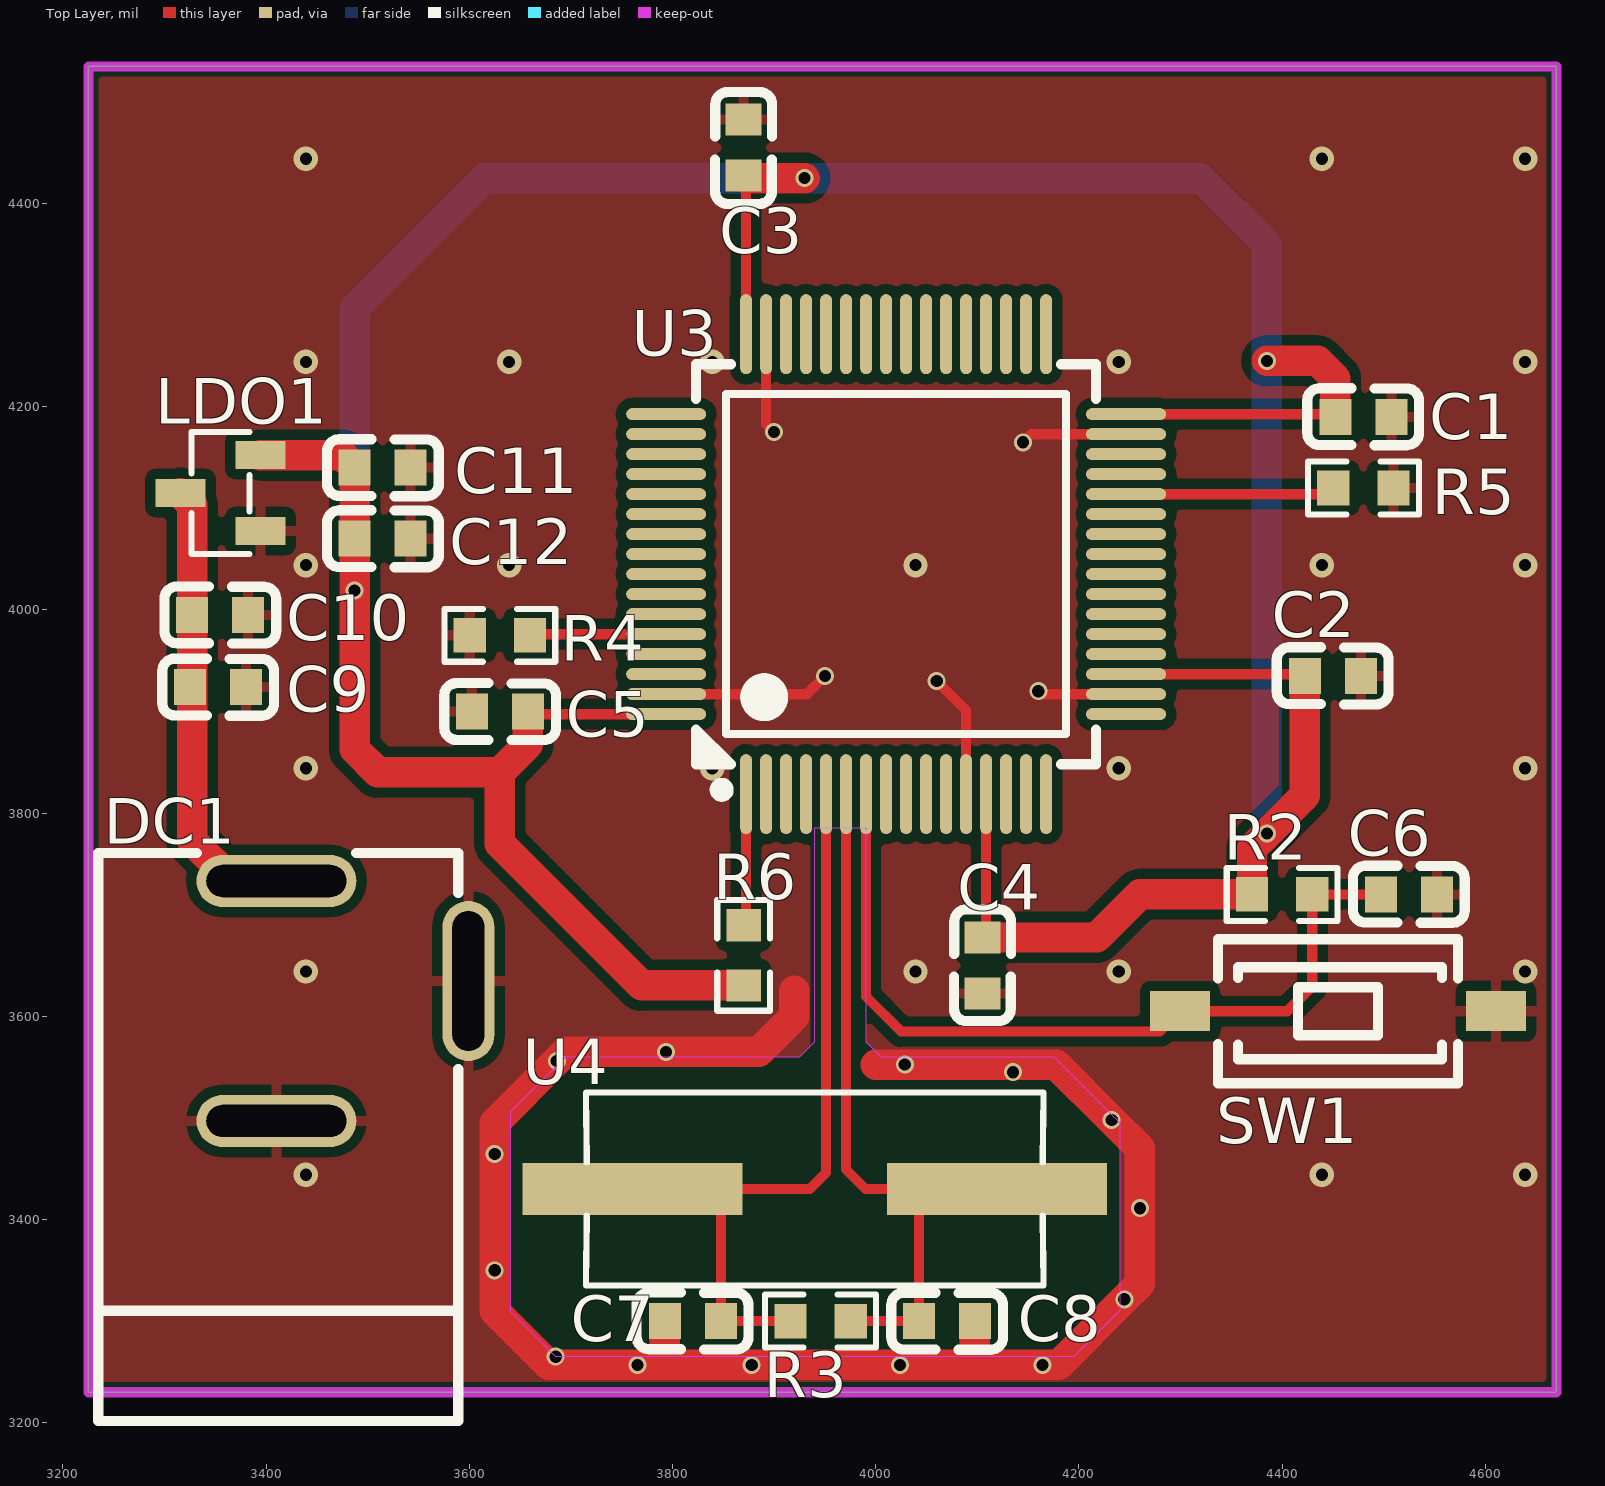
[diagram p0: Top Layer view]
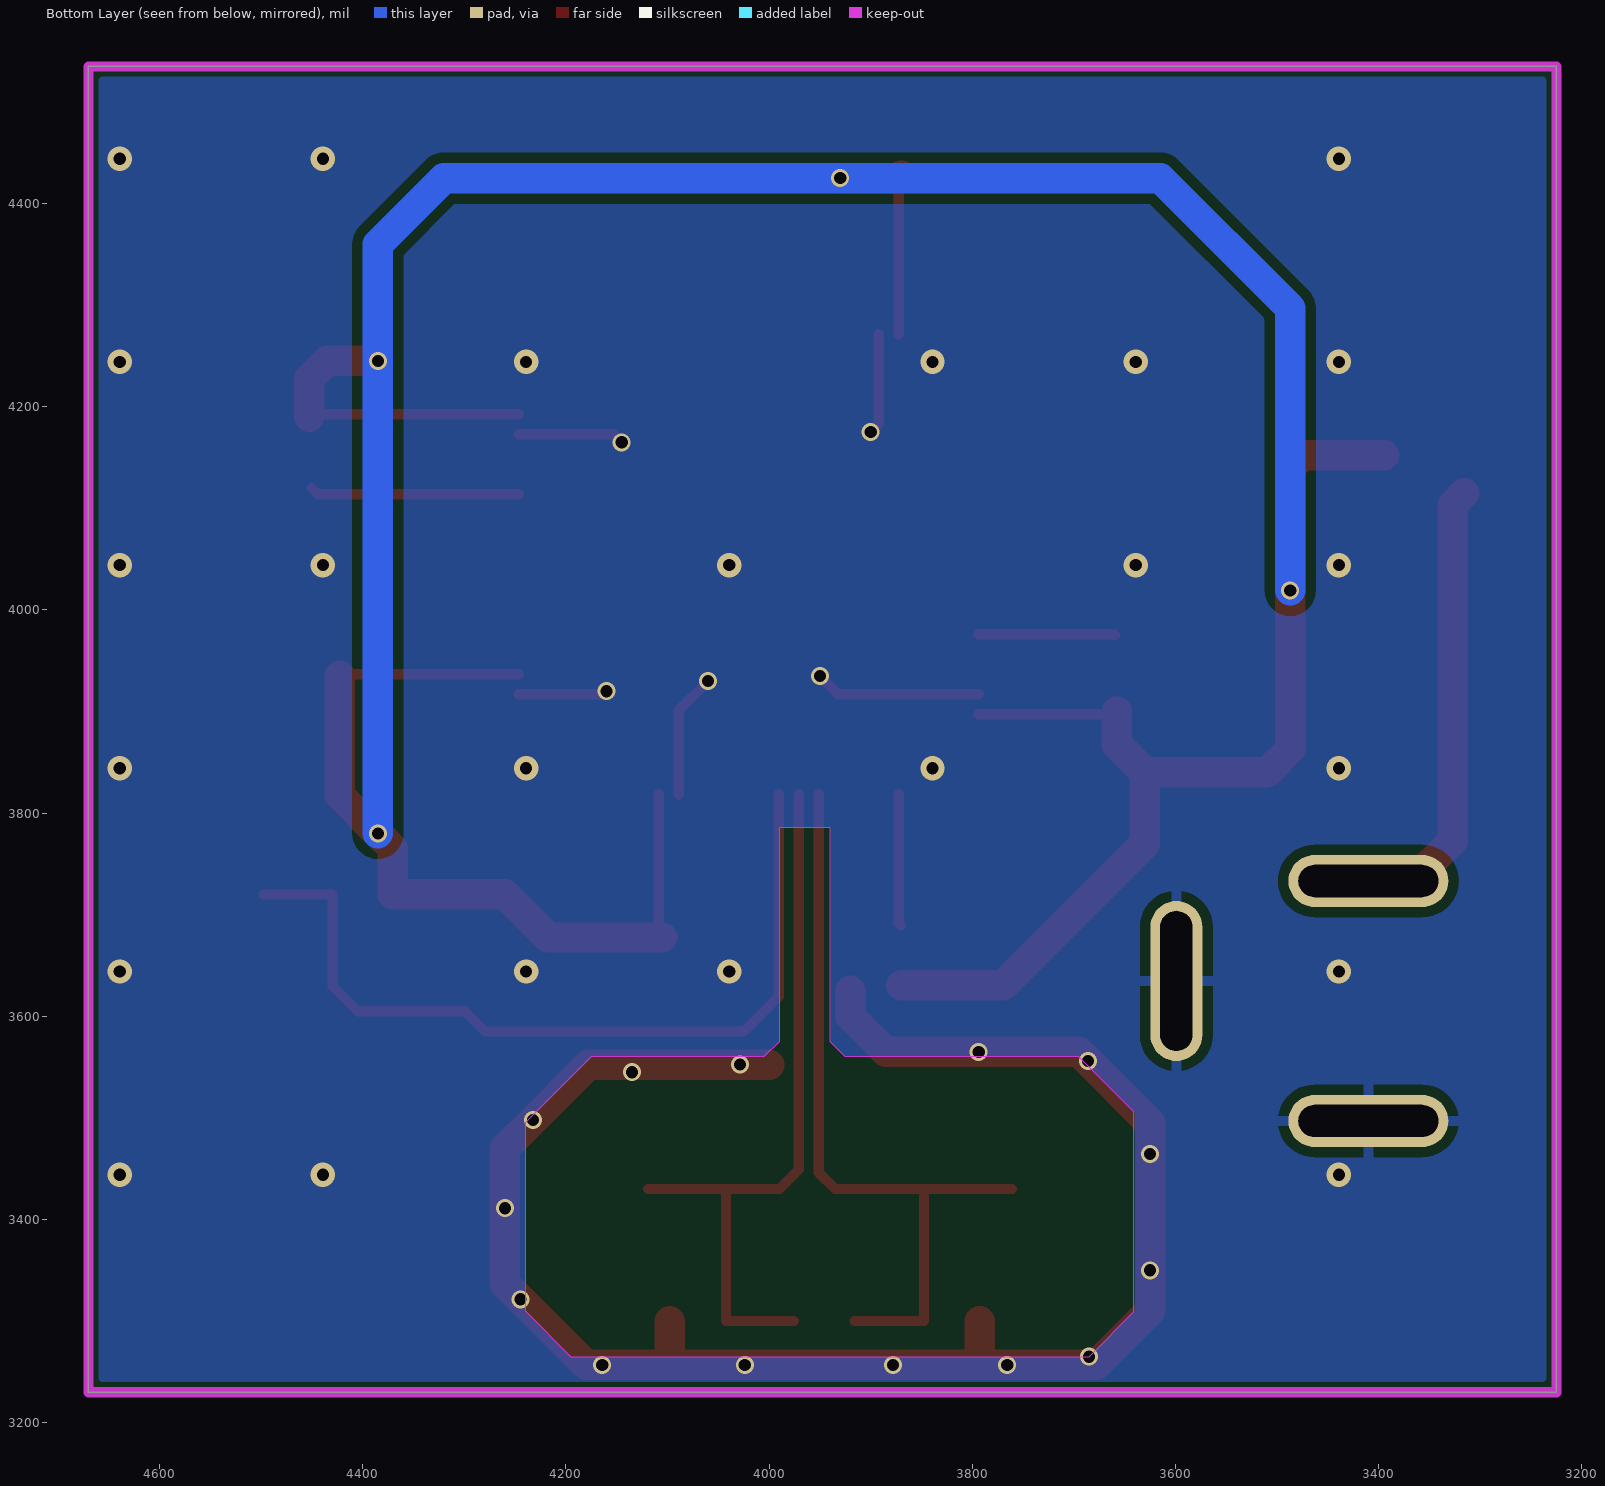
[diagram p1: Bottom Layer view, seen from below]
# Altium PCB MISC52126.pcbdoc
Units mil, origin at the board's own origin, x right, y up, seen from the top; angles counter-clockwise.
Board outline 1445 x 1305 mil, 2 copper layers (Top Layer, Bottom Layer), stack 62.206 mil thick; 22 components, 57 nets, 108 pads, 47 vias.

## Layer stack, top to bottom
Top Solder Mask Layer: solder mask 0.394, Dk 3.3
Top Layer: signal copper 1.379
Dielectric1: surface 59.449, FR4, Dk 4.5
Bottom Layer: signal copper 1.378
Bottom Solder Mask Layer: solder mask 0.394, Dk 3.3

## Board outline
3225,4535 3225,3230 4670,3230 4670,4535

## Design rules (kind name [scope] priority, off if disabled: settings)
BoardOutlineClearance copperThickness2oz_1 [All] p2 off: genericclearance=7.99 ignorepadtopadclearanceinfootprint=FALSE except(0: Arc-SplitContinuation Track-SplitContinuation SMDPad-SplitContinuation THPad-SplitContinuation Via-SplitContinuation Fill-SplitContinuation Region-SplitContinuation Poly-SplitContinuation Text-SplitContinuation Hole-SplitContinuation; 5.98: Arc-CutoutEdge Track-CutoutEdge SMDPad-CutoutEdge THPad-CutoutEdge Via-CutoutEdge Fill-CutoutEdge Region-CutoutEdge Text-CutoutEdge Hole-CutoutEdge; 10: Poly-OutlineEdge Poly-CutoutEdge; 11.81: Arc-OutlineEdge Track-OutlineEdge SMDPad-OutlineEdge THPad-OutlineEdge Via-OutlineEdge Fill-OutlineEdge Region-OutlineEdge Text-OutlineEdge Hole-OutlineEdge)
BoardOutlineClearance Plane_innerPlane_1 [All] p4 off: genericclearance=4.02 ignorepadtopadclearanceinfootprint=FALSE except(0: Arc-SplitContinuation Track-SplitContinuation SMDPad-SplitContinuation THPad-SplitContinuation Via-SplitContinuation Fill-SplitContinuation Region-SplitContinuation Poly-SplitContinuation Text-SplitContinuation Hole-SplitContinuation; 5.98: Arc-CutoutEdge Track-CutoutEdge SMDPad-CutoutEdge THPad-CutoutEdge Via-CutoutEdge Fill-CutoutEdge Region-CutoutEdge Text-CutoutEdge Hole-CutoutEdge; 10: Poly-OutlineEdge Poly-CutoutEdge; 11.81: Arc-OutlineEdge Track-OutlineEdge SMDPad-OutlineEdge THPad-OutlineEdge Via-OutlineEdge Fill-OutlineEdge Region-OutlineEdge Text-OutlineEdge Hole-OutlineEdge)
BoardOutlineClearance Copper_copperRegion_1 [All] p6 off: genericclearance=4.02 ignorepadtopadclearanceinfootprint=FALSE except(0: Arc-SplitContinuation Track-SplitContinuation SMDPad-SplitContinuation THPad-SplitContinuation Via-SplitContinuation Fill-SplitContinuation Region-SplitContinuation Poly-SplitContinuation Text-SplitContinuation Hole-SplitContinuation; 5.98: Arc-CutoutEdge Track-CutoutEdge SMDPad-CutoutEdge THPad-CutoutEdge Via-CutoutEdge Fill-CutoutEdge Region-CutoutEdge Text-CutoutEdge Hole-CutoutEdge; 10: Poly-OutlineEdge Poly-CutoutEdge; 11.81: Arc-OutlineEdge Track-OutlineEdge SMDPad-OutlineEdge THPad-OutlineEdge Via-OutlineEdge Fill-OutlineEdge Region-OutlineEdge Text-OutlineEdge Hole-OutlineEdge)
BoardOutlineClearance copperThickness1oz_1 [All] p8: genericclearance=4.02 ignorepadtopadclearanceinfootprint=FALSE except(0: Arc-SplitContinuation Track-SplitContinuation SMDPad-SplitContinuation THPad-SplitContinuation Via-SplitContinuation Fill-SplitContinuation Region-SplitContinuation Poly-SplitContinuation Text-SplitContinuation Hole-SplitContinuation; 5.98: Arc-CutoutEdge Track-CutoutEdge SMDPad-CutoutEdge THPad-CutoutEdge Via-CutoutEdge Fill-CutoutEdge Region-CutoutEdge Text-CutoutEdge Hole-CutoutEdge; 10: Poly-OutlineEdge Poly-CutoutEdge; 11.81: Arc-OutlineEdge Track-OutlineEdge SMDPad-OutlineEdge THPad-OutlineEdge Via-OutlineEdge Fill-OutlineEdge Region-OutlineEdge Text-OutlineEdge Hole-OutlineEdge)
Clearance copperThickness2oz [All] p1 off: gap=7.99 ignorepadtopadclearanceinfootprint=FALSE except(5.98: SMDPad-Track SMDPad-SMDPad THPad-Track SMDPad-THPad THPad-THPad Track-Via SMDPad-Via THPad-Via Via-Via Fill-Track Region-Track Fill-SMDPad Region-SMDPad Fill-THPad Region-THPad Fill-Via Region-Via Fill-Fill Fill-Region Region-Region Arc-Track Arc-SMDPad Arc-THPad Arc-Via Fill-Arc Region-Arc Arc-Arc Text-Track SMDPad-Text Text-THPad Text-Via Fill-Text Region-Text Arc-Text Text-Text Hole-Track Hole-SMDPad Hole-THPad Hole-Via Fill-Hole Region-Hole Hole-Arc Hole-Text; 10: Poly-Track Poly-SMDPad Poly-THPad Poly-Via Poly-Fill Poly-Region Poly-Poly Poly-Arc Poly-Text Poly-Hole)
Clearance Plane_innerPlane [All] p3 off: gap=4.02 ignorepadtopadclearanceinfootprint=FALSE except(5.98: SMDPad-Track SMDPad-SMDPad THPad-Track SMDPad-THPad THPad-THPad Track-Via SMDPad-Via THPad-Via Via-Via Fill-Track Region-Track Fill-SMDPad Region-SMDPad Fill-THPad Region-THPad Fill-Via Region-Via Fill-Fill Fill-Region Region-Region Arc-Track Arc-SMDPad Arc-THPad Arc-Via Fill-Arc Region-Arc Arc-Arc Text-Track SMDPad-Text Text-THPad Text-Via Fill-Text Region-Text Arc-Text Text-Text Hole-Track Hole-SMDPad Hole-THPad Hole-Via Fill-Hole Region-Hole Hole-Arc Hole-Text; 10: Poly-Track Poly-SMDPad Poly-THPad Poly-Via Poly-Fill Poly-Region Poly-Poly Poly-Arc Poly-Text Poly-Hole)
Clearance Copper_copperRegion [All] p5 off: gap=4.02 ignorepadtopadclearanceinfootprint=FALSE except(5.98: SMDPad-Track SMDPad-SMDPad THPad-Track SMDPad-THPad THPad-THPad Track-Via SMDPad-Via THPad-Via Via-Via Fill-Track Region-Track Fill-SMDPad Region-SMDPad Fill-THPad Region-THPad Fill-Via Region-Via Fill-Fill Fill-Region Region-Region Arc-Track Arc-SMDPad Arc-THPad Arc-Via Fill-Arc Region-Arc Arc-Arc Text-Track SMDPad-Text Text-THPad Text-Via Fill-Text Region-Text Arc-Text Text-Text Hole-Track Hole-SMDPad Hole-THPad Hole-Via Fill-Hole Region-Hole Hole-Arc Hole-Text; 10: Poly-Track Poly-SMDPad Poly-THPad Poly-Via Poly-Fill Poly-Region Poly-Poly Poly-Arc Poly-Text Poly-Hole)
Clearance copperThickness1oz [All] p7: gap=4.02 ignorepadtopadclearanceinfootprint=FALSE except(5.98: SMDPad-Track SMDPad-SMDPad THPad-Track SMDPad-THPad THPad-THPad Track-Via SMDPad-Via THPad-Via Via-Via Fill-Track Region-Track Fill-SMDPad Region-SMDPad Fill-THPad Region-THPad Fill-Via Region-Via Fill-Fill Fill-Region Region-Region Arc-Track Arc-SMDPad Arc-THPad Arc-Via Fill-Arc Region-Arc Arc-Arc Text-Track SMDPad-Text Text-THPad Text-Via Fill-Text Region-Text Arc-Text Text-Text Hole-Track Hole-SMDPad Hole-THPad Hole-Via Fill-Hole Region-Hole Hole-Arc Hole-Text; 10: Poly-Track Poly-SMDPad Poly-THPad Poly-Via Poly-Fill Poly-Region Poly-Poly Poly-Arc Poly-Text Poly-Hole)
DiffPairsRouting differentialPair [All] p1: maxlimit=6 minlimit=6 mostfreqgap=6 toplayer_minwidth=5 toplayer_prefwidth=10 toplayer_maxwidth=100 toplayer_mingap=6 toplayer_prefgap=6 toplayer_maxgap=6 bottomlayer_minwidth=5 bottomlayer_prefwidth=10 bottomlayer_maxwidth=100 bottomlayer_mingap=6 bottomlayer_prefgap=6 bottomlayer_maxgap=6 maxuncoupledlength=10
HoleToHoleClearance otherClearance [All] p1: gap=11.8 allowstackedmicrovias=TRUE
Length netLength [All] p1: minlimit=0 maxlimit=0
PasteMaskExpansion pasteMaskExpansion [All] p1: expansion=0
PlaneConnect innerPlane [All] p1: planeconnectstyle=Relief reliefexpansion=20 reliefentries=4 reliefconductorwidth=10 reliefairgap=10
PolygonConnect copperRegion [(InNet('GND'))] p1: connectstyle=Relief reliefconductorwidth=10 reliefentries=4 polygonreliefangle="90 Angle" airgapwidth=10 via.connectstyle=Relief via.reliefconductorwidth=10 via.reliefentries=4 via.polygonreliefangle="90 Angle" via.airgapwidth=10
RoutingVias viaSize [All] p1: holewidth=12.01 width=24.02 viastyle="Through Hole" minholewidth=11.81 minwidth=17.72 maxholewidth=248.03 maxwidth=393.7
SolderMaskExpansion solderMaskExpansion [IsVia] p1: expansion=-1000 istentingtop=TRUE
SolderMaskExpansion solderMaskExpansion [All] p2: expansion=2.01 istentingtop=FALSE
Width copperThickness2oz_2 [All] p1 off: maxlimit=100 minlimit=8 preferedwidth=10
Width copperThickness1oz_2 [All] p2: maxlimit=100 minlimit=5 preferedwidth=10

## Components (designator, comment, footprint, x,y, rotation, side; value= is the part's Value field where it differs from the comment)
C1 "100nF" C0603 4480,4190 r0 top
C2 "100nF" C0603 4450,3935 r0 top
C3 "100nF" C0603 3870,4455 r90 top
C4 "100nF" C0603 4105,3650 r270 top
C5 "100nF" C0603 3630,3900 r180 top
C6 "100nF" C0603 4525,3720 r0 top
C7 "22pf" C0603 3820,3300 r0 top
C8 "22pf" C0603 4070,3300 r180 top
C9 "10uF" C0603 3352.53,3924.04 r180 top
C10 "100nF" C0603 3354.63,3995.07 r180 top
C11 "100nF" C0603 3514.63,4140.07 r180 top
C12 "10uF" C0603 3514.63,4070.07 r180 top
DC1 "" DC-2.0 3399.63,3610.07 r270 top
LDO1 "SC662K-3.3V" SOT-23-3_L2.9-W1.3-P1.90-LS2.4-BR 3355,4115 r0 top
R2 "10K" R0603 4400,3720 r0 top
R3 "1M" R0603 3945.68,3300 r180 top
R4 "0" R0603 3630,3975 r180 top
R5 "0" R0603 4480,4120 r0 top
R6 "0" R0603 3870,3660 r90 top
SW1 "SMD push button ANJIAN_2PIN" SW-SMD_L6.0-W3.6-LS8.0 4455,3605 r0 top
U3 "STM32F103RCT6TR" LQFP-64_L10.0-W10.0-P0.50-LS12.0-BL 4020,4045 r0 top
U4 "Crystal 8M-HC-49S/SMD" HC-49S_L11.4-W4.8-LS12.7 3940,3430 r0 top

## Footprints (in the part's own frame and the unit in brackets; to place one, negate y for a bottom-side part, rotate by r counter-clockwise, add the part's x,y. Pads: shape width x height; smd on the part's side, far side on the other; paste and mask are expansions set on the pad)
C0603 [mm]
  rect 0.8x0.9 smd paste+0 mask+0.051: 1(-0.7,0) 2(0.7,0)
  silkscreen extent -1.41,-0.71 1.39,0.72
DC-2.0 [mil]
  oval 157.5x51.2 hole 31.5 slot 137.8 at 0 deg paste+0 mask+2: 2(-24.7,199.5)
  oval 51.2x157.5 hole 31.5 slot 137.8 at 90 deg paste+0 mask+2: 3(113.1,10.5) 4(-123.1,10.5)
  silkscreen extent -151,-165 408,190
HC-49S_L11.4-W4.8-LS12.7 [mm]
  rect 5.5x1.3 smd paste+0 mask+0.051: 1(-4.553,0) 2(4.553,0)
  silkscreen extent -5.71,-2.41 5.71,2.41
LQFP-64_L10.0-W10.0-P0.50-LS12.0-BL [mm]
  oval 0.3x2 smd paste+0 mask+0.051: 1(-3.75,-5.75) 2(-3.25,-5.75) 3(-2.75,-5.75) 4(-2.25,-5.75) 5(-1.75,-5.75) 6(-1.25,-5.75) 7(-0.75,-5.75) 8(-0.25,-5.75) 9(0.25,-5.75) 10(0.75,-5.75) 11(1.25,-5.75) 12(1.75,-5.75) 13(2.25,-5.75) 14(2.75,-5.75) 15(3.25,-5.75) 16(3.75,-5.75) 33(3.75,5.75) 34(3.25,5.75) 35(2.75,5.75) 36(2.25,5.75) 37(1.75,5.75) 38(1.25,5.75) 39(0.75,5.75) 40(0.25,5.75) 41(-0.25,5.75) 42(-0.75,5.75) 43(-1.25,5.75) 44(-1.75,5.75) 45(-2.25,5.75) 46(-2.75,5.75) 47(-3.25,5.75) 48(-3.75,5.75)
  oval 2x0.3 smd paste+0 mask+0.051: 17(5.75,-3.75) 18(5.75,-3.25) 19(5.75,-2.75) 20(5.75,-2.25) 21(5.75,-1.75) 22(5.75,-1.25) 23(5.75,-0.75) 24(5.75,-0.25) 25(5.75,0.25) 26(5.75,0.75) 27(5.75,1.25) 28(5.75,1.75) 29(5.75,2.25) 30(5.75,2.75) 31(5.75,3.25) 32(5.75,3.75) 49(-5.75,3.75) 50(-5.75,3.25) 51(-5.75,2.75) 52(-5.75,2.25) 53(-5.75,1.75) 54(-5.75,1.25) 55(-5.75,0.75) 56(-5.75,0.25) 57(-5.75,-0.25) 58(-5.75,-0.75) 59(-5.75,-1.25) 60(-5.75,-1.75) 61(-5.75,-2.25) 62(-5.75,-2.75) 63(-5.75,-3.25) 64(-5.75,-3.75)
  silkscreen extent -5,-5.79 5,5
R0603 [mil]
  rect 31.75x34.02 smd paste-3937.01 mask+2: 1(-29.66,0) 2(29.66,0)
  silkscreen extent -55,-26 55,26
SOT-23-3_L2.9-W1.3-P1.90-LS2.4-BR [mm]
  rect 1.25x0.7 smd: 1(1,-0.95) 2(1,0.95) 3(-1,0)
  silkscreen extent -0.73,-1.53 0.73,1.53
SW-SMD_L6.0-W3.6-LS8.0 [mm]
  rect 1.5x1 smd paste+0 mask+0.051: 1(-3.95,0) 2(3.95,0)
  silkscreen extent -3,-1.8 3,1.8

## Via types
v1: diameter 24.02, hole 12, Top Layer to Bottom Layer, 24 vias
v2: diameter 17.72, hole 12, Top Layer to Bottom Layer, 23 vias

## Nets (pads, with @x,y where several pads share a name; then routed paths per layer and width w, separated by ;. In a path a pad name is that pad's centre, name@x,y a point inside that pad or via, vN(x,y) a via of type N, cw(c..) or ccw(c..) an arc to the next point about the centre after c; other vN are vias at no path point)
+5V: C9.2 C10.2 DC1.4 LDO1.3 | length 446.3
  Top Layer w30: LDO1.3 3327.07,4103.56 C10.2 3327.07,3772.93 3366.83,3733.17 DC1.4
BOOT0: R4.1 U3.60 | length 134.4
  Top Layer w10: R4.1 3660.76,3976.1 U3.60
BOOT1: R5.1 U3.28 | length 206.5
  Top Layer w10: U3.28 4444.24,4113.9 R5.1
GND: C1.2 C2.2 C3.2 C4.2 C5.2 C6.2 C7.1 C8.1 C9.1 C10.1 C11.1 C12.1 DC1.2 DC1.3 LDO1.1 R4.2 R5.2 SW1.2 U3.12 U3.18 U3.31 U3.47 U3.63 | length 2335
  Top Layer w10: U3.63 3932.05,3917.05 v2(3950,3935) ; U3.47 3892.05,4182.95 v2(3900,4175) ; v2(4060,3930) 4088.9,3901.1 U3.12 ; v2(4145,4165) 4152.95,4172.95 U3.31 ; v2(4160,3920) 4162.95,3917.05 U3.18
  Top Layer w30: C7.1 3792.44,3259.95 3789.3,3256.81 ; 3920,3625 3920,3600 3885,3565 v2(3793.69,3565) 3695,3565 v2(3686.13,3556.13) 3625,3495 v2(3625,3464.47) v2(3625,3350) 3625,3310 3678.19,3256.81 v2(3765.62,3256.81) 3789.3,3256.81 ; 4000,3552.5 v2(4028.56,3552.5) 4177.5,3552.5 v2(4232.2,3497.8) 4260,3470 v2(4260,3411.13) 4260,3336.81 v2(4244.6,3321.41) 4180,3256.81 v2(4164.24,3256.81) 4092.09,3256.81 ; C8.1 4097.56,3262.28 4092.09,3256.81 ; 3789.3,3256.81 v2(3877.91,3256.81) v2(4023.88,3256.81) 4092.09,3256.81
  other v1: 3439.1,3444.1 4439.1,3444.1 4639.1,3444.1 3439.1,3644.1 4039.1,3644.1 4239.1,3644.1 4639.1,3644.1 3439.1,3844.1 3839.1,3844.1 4239.1,3844.1 4639.1,3844.1 3439.1,4044.1 3639.1,4044.1 4039.1,4044.1 4439.1,4044.1 4639.1,4044.1 3439.1,4244.1 3639.1,4244.1 3839.1,4244.1 4239.1,4244.1 4639.1,4244.1 3439.1,4444.1 4439.1,4444.1 4639.1,4444.1
  other v2: 3685,3265 4135,3545
OSC_IN: C7.2 R3.2 U3.5 U4.1 | length 768
  Top Layer w10: U4.1 U4.1@3847.56,3430 ; R3.2 C7.2 U4.1@3847.56,3430 ; U3.5 3951.1,3446.1 3935,3430 U4.1@3847.56,3430
OSC_OUT: C8.2 R3.1 U3.6 U4.2 | length 722.9
  Top Layer w10: U3.6 3970.79,3449.21 3990,3430 U4.2@4042.44,3430 ; R3.1 C8.2 U4.2@4042.44,3430 ; U4.2 U4.2@4042.44,3430
PA0: U3.14
PA1: U3.15
PA2: U3.16
PA3: U3.17
PA4: U3.20
PA5: U3.21
PA6: U3.22
PA7: U3.23
PA8: U3.41
PA9: U3.42
PA10: U3.43
PA11: U3.44
PA12: U3.45
PA13: U3.46
PA14: U3.49
PA15: U3.50
PB0: U3.26
PB1: U3.27
PB3: U3.55
PB4: U3.56
PB5: U3.57
PB6: U3.58
PB7: U3.59
PB8: U3.61
PB9: U3.62
PB10: U3.29
PB11: U3.30
PB12: U3.33
PB13: U3.34
PB14: U3.35
PB15: U3.36
PC0: U3.8
PC1: U3.9
PC2: U3.10
PC3: U3.11
PC4: U3.24
PC5: U3.25
PC6: U3.37
PC7: U3.38
PC8: U3.39
PC9: U3.40
PC10: U3.51
PC11: U3.52
PC12: U3.53
PC13: U3.2
PC14: U3.3
PC15: U3.4
PD2: U3.54
RST: C6.1 R2.2 SW1.1 U3.7 | length 829.2
  Top Layer w10: U3.7 3990.47,3619.53 4025,3585 4279.49,3585 SW1.1 4405,3605 4429.66,3629.66 R2.2 C6.1
VBAT: R6.2 U3.1 | length 129.9
  Top Layer w10: R6.2 3872.36,3692.02 U3.1
VCC: C1.1 C2.1 C3.1 C4.1 C5.1 C11.2 C12.2 LDO1.2 R2.1 R6.1 U3.13 U3.19 U3.32 U3.48 U3.64 | length 4312.5
  Top Layer w10: C5.1 3660.2,3897.36 U3.64 ; U3.48 C3.1@3872.36,4425.08 ; C4.1 4108.58,3681.14 U3.13 ; U3.19 4420.71,3936.73 C2.1 ; U3.32 4449.8,4192.64 C1.1
  Top Layer w30: LDO1.2 3474.74,4152.4 C11.2 C12.2 v2(3487.07,4019.16) 3487.07,3862.93 3510,3840 3630,3840 ; C5.1 3657.56,3867.56 3630,3840 ; R6.1 3769.66,3630.34 3630,3770 3630,3840 ; C3.1 3872.36,4425.08 3872.44,4425 v2(3930,4425) ; C4.1 4217.56,3677.56 4260,3720 R2.1 4370.34,3765.34 v2(4385,3780) 4422.44,3817.44 C2.1 ; v2(4385,4245) 4435,4245 4452.44,4227.56 C1.1
  Bottom Layer w30: v2(3487.07,4019.16) 3487.07,4297.07 3615,4425 v2(3930,4425) 4320,4425 4385,4360 v2(4385,4245) v2(4385,3780)

## Polygon pours and split planes (outlines as drawn)
GND on Top Layer (solid, remove dead copper, pour order 2): 3060,4685 3060,3000 4885,3000 4885,4685
GND on Bottom Layer (solid, remove dead copper, pour order 2): 3000,4650 3000,3060 4730,3060 4730,4650

## Keep-outs
Board Outline Layer:
  region: 3940,3785.65 3989.27,3785.65 3990.47,3784.45 3990,3783.98 3990,3575 4005,3560 4175,3560 4240,3495 4240,3310 4195,3265 3685,3265 3640.83,3309.17 3640.83,3505.83 3695,3560 3925,3560 3940,3575
  lines w10: 3225,3230 3225,4535 4670,4535 4670,3230 3225,3230